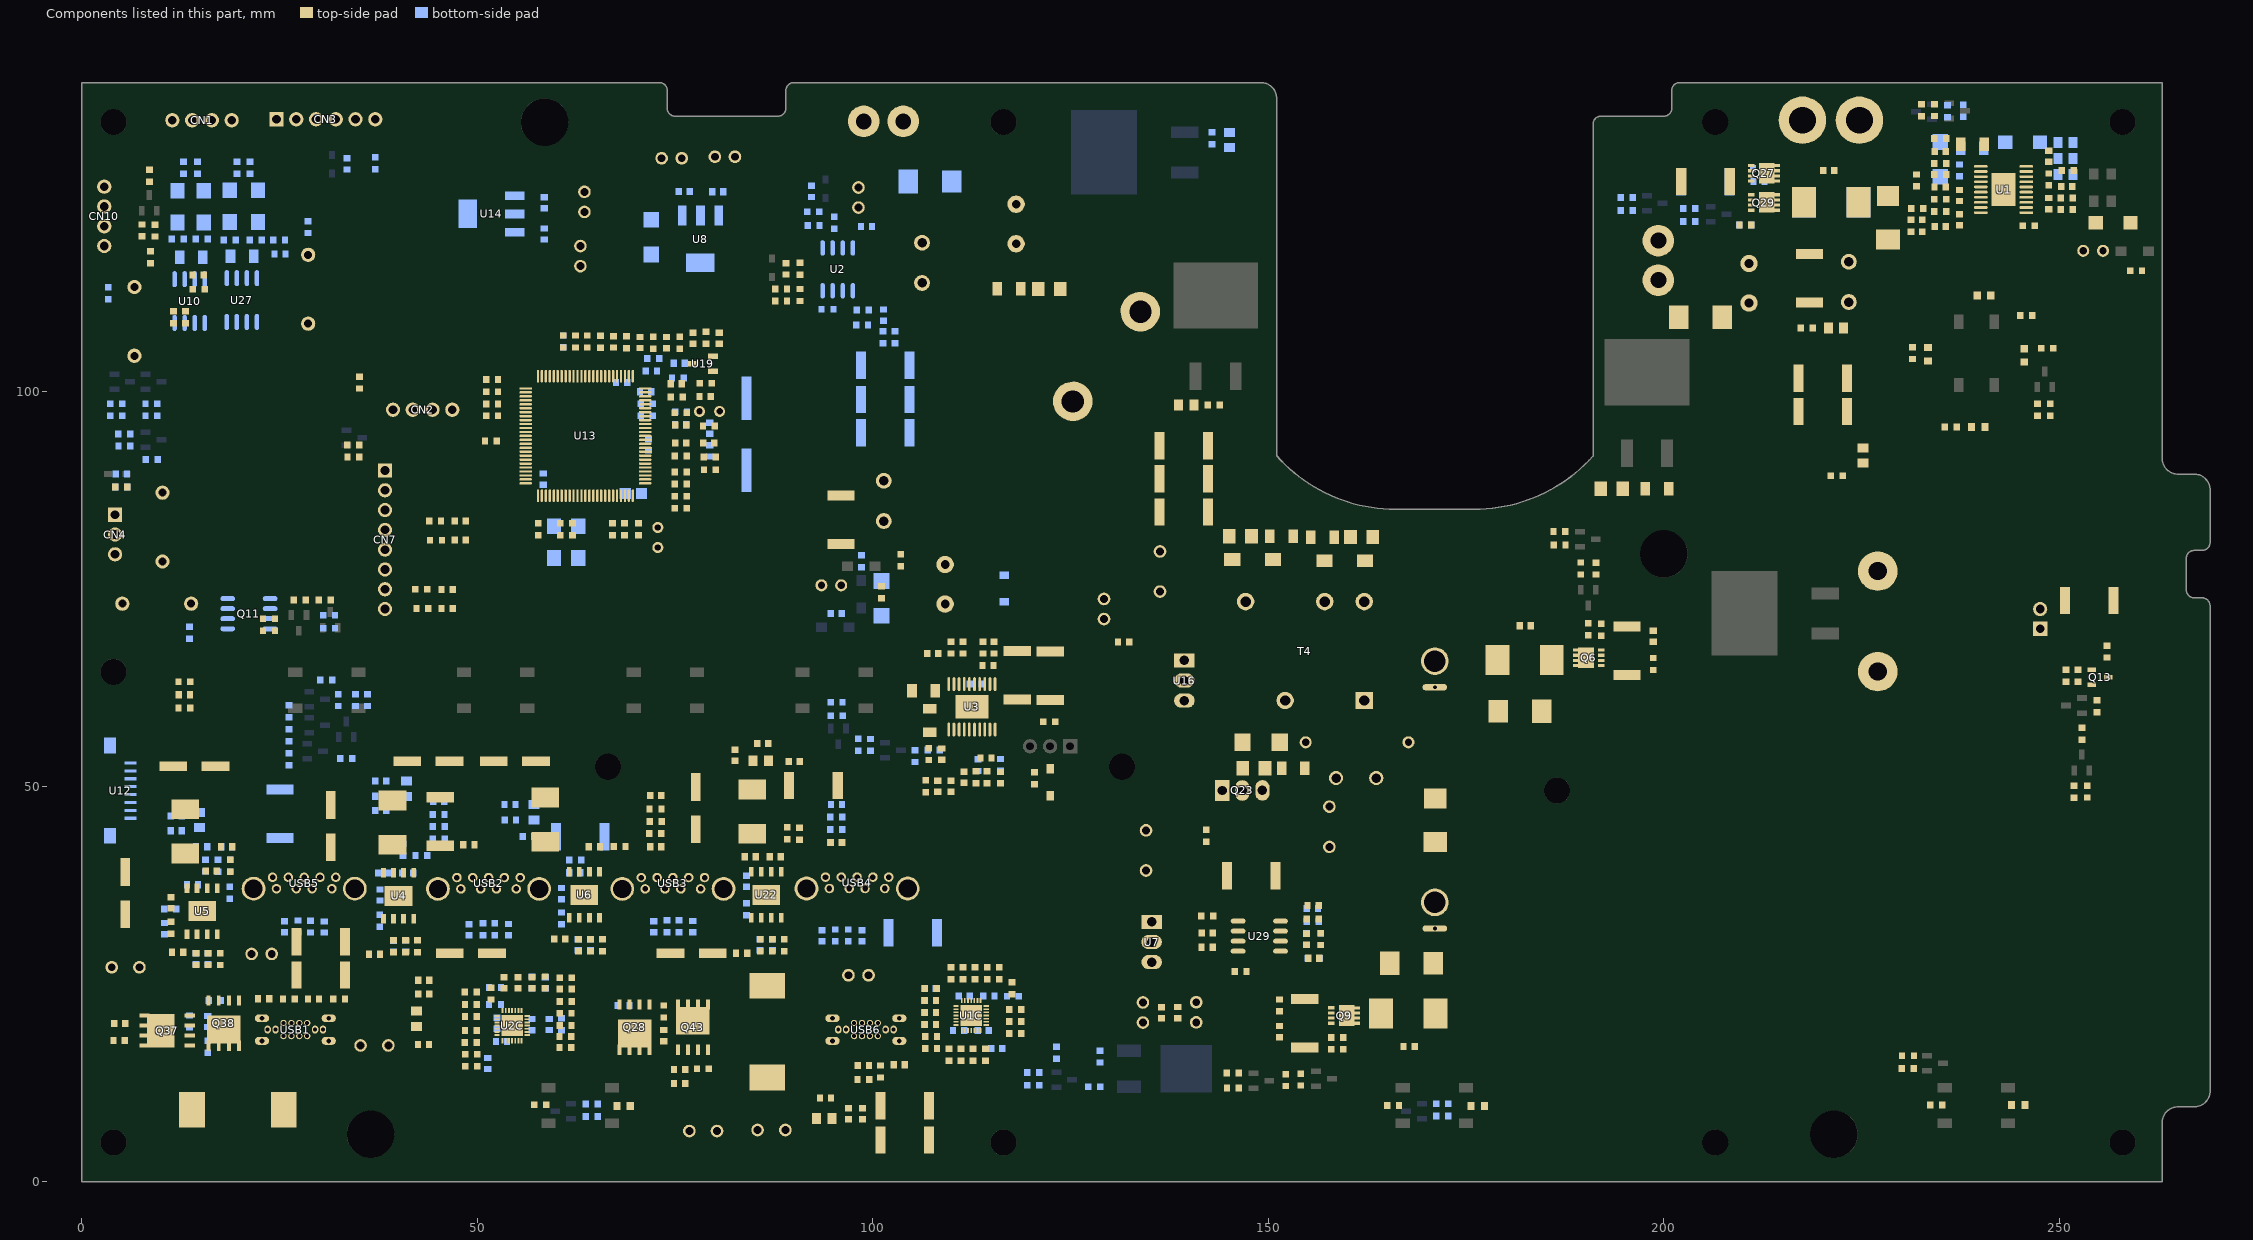
[diagram p0: the components of this part, seen from the top]
# Altium PCB MISC84402.PcbDoc (part 2 of 12)
Units mm, origin at the board's own origin, x right, y up, seen from the top; angles counter-clockwise.
Board outline 269.06 x 139 mm, 4 copper layers (TOP, GND02, PWR03, BOTTOM), stack 0.732 mm thick; 694 components, 428 nets, 1859 pads, 1384 vias.

## Components (designator, comment, footprint, x,y, rotation, side; value= is the part's Value field where it differs from the comment) (continued)
R13 "AC2512FK-073KL" R2512 118.238,64.049 r270 top
R14 "" R0603 113.03,51.181 r270 top
R15 "" R0603 109.855,67.564 r270 top
R16 "15K" RES-TH_BD3.3-L9.0-P13.00-D0.6 161.212,55.591 r0 top
R17 "1K" R0603 45.085,46.441 r0 bottom
R18 "0.01" R2512 220.109,97.409 r180 top
R19 "" RES-SMD_L6.4-W3.2-R2512 195.334,67.157 r0 top
R20 "49.9K" R0603 120.447,51.044 r90 top
R21 "" R0603 246.126,120.904 r180 top
R22 "" R0603 113.919,67.564 r270 top
R23 "2K" R0603 154.102,12.944 r90 top
R24 "1K" R0603 45.102,44.923 r180 bottom
R25 "" R0603 115.316,67.564 r270 top
R26 "" R2512 205.263,126.496 r0 top
R27 "" R0603 250.943,124.398 r180 top
R28 "" R2512 45.289,45.583 r90 top
R29 "" R0603 152.187,12.886 r270 top
R30 "1K" R0603 18.695,36.549 r90 bottom
R31 "" R2512 25.045,46.574 r90 bottom
R32 "2K" R0603 145.5,13.777 r0 top
R33 "" R0603 79.4,90.053 r0 top
R34 "" R0603 232.029,123.063 r0 top
R35 "2K" R0603 189.484,77.562 r90 top
R36 "" R0603 60.858,106.274 r270 bottom
R37 "" R0603 107.696,54.61 r0 bottom
R38 "" R0603 3.328,112.36 r90 bottom
R39 "" R0603 191.439,77.556 r90 top
R40 "2K" R0603 186.813,80.544 r0 top
R41 "" R2512 139.323,84.709 r0 top
R42 "" R0603 23.648,69.688 r180 top
R43 "" R0603 113.021,62.941 r180 bottom
R44 "" R0603 186.795,82.219 r180 top
R45 "" R2512 205.237,126.446 r0 bottom
R46 "" R0603 79.274,95.596 r0 top
R47 "1K" R0603 62.002,82.523 r90 top
R48 "" R0603 259.7,115.215 r180 top
R49 "" R0603 250.943,122.936 r180 top
R50 "AC2512FK-073KL" R2512 122.428,64.018 r90 top
R51 "2K" R0603 105.308,53.848 r90 bottom
R52 "" R0603 234.95,127.381 r0 top
R53 "" R0603 95.428,58.953 r0 bottom
R54 "" R1206 107.188,58.359 r90 top
R55 "" R0603 251.07,127.889 r180 top
R56 "" R0603 210.312,120.98 r0 top
R57 "100K" NTC 72.806,81.484 r90 top
R58 "1K" R0603 72.543,45.558 r0 top
R59 "" R2512 105.054,31.506 r180 bottom
R60 "" R0603 210.301,120.99 r0 bottom
R61 "" R0603 158.722,16.779 r180 top
R62 "1K" R0603 72.517,47.152 r180 top
R63 "" R0603 18.745,40.006 r270 bottom
R64 "2K" R0603 234.442,9.728 r0 top
R65 "10K" R0603 145.515,11.887 r180 top
R66 "" R0603 190.444,69.865 r270 top
R67 "1K" R0603 212.025,128.153 r0 bottom
R68 "" R0603 252.375,64.012 r90 top
R69 "1K" R0603 151.41,22.317 r270 top
R70 "1K" R0603 198.654,65.488 r90 top
R71 "" R0603 250.851,64.003 r90 top
R72 "" R0603 158.722,18.253 r0 top
R73 "2K" R0603 95.402,60.655 r180 bottom
R74 "" R0805 145.11,132.029 r270 bottom
R75 "" R0603 88.392,111.379 r180 top
R76 "" R0603 45.093,43.342 r180 bottom
R77 "1K" R0603 11.183,34.518 r0 bottom
R78 "2K" R0603 248.463,105.41 r0 top
R79 "2K" R0603 231.445,104.8 r270 top
R80 "" R0603 71.4,96.866 r180 bottom
R81 "100" R0603 40.92,29.818 r90 top
R82 "" R2512 63.018,43.653 r180 bottom
R83 "" R2512 92.482,50.13 r180 top
R84 "100" R0603 73.965,32.334 r90 bottom
R85 "1K" R0603 95.377,42.926 r180 bottom
R86 "" R0603 78.892,106.731 r90 top
R87 "" R0603 72.491,44.054 r0 top
R88 "36K" R0603 60.639,19.947 r90 bottom
R89 "100" R0603 39.396,29.818 r90 top
R90 "100" R0603 75.489,32.343 r90 bottom
R91 "" R0603 4.335,98.39 r180 bottom
R92 "100" R0603 28.905,32.292 r90 bottom
R93 "" R0603 8.789,98.39 r180 bottom
R94 "" R0603 51.85,98.339 r0 top
R95 "" R0603 36.094,60.925 r270 bottom
R96 "" R0603 95.352,44.552 r0 bottom
R97 "100" R0603 27.331,32.3 r90 bottom
R98 "2K" R0603 27.525,73.558 r0 top
R99 "1K" R0603 95.377,46.126 r0 bottom
R100 "10K" R0603 30.709,73.558 r180 top
R101 "" R0805 139.903,98.222 r180 top
R102 "100" R0603 52.197,31.957 r90 bottom
R103 "1K" R0603 18.745,39.999 r90 top
R104 "10K" R0603 98.146,55.27 r270 bottom
R105 "" R0603 5.368,93.056 r0 bottom
R106 "" R2512 101.582,98.933 r180 bottom
R107 "" R0603 90.805,115.443 r270 top
R108 "" R2512 101.582,94.742 r180 bottom
R109 "" R2512 101.582,103.251 r180 bottom
R110 "0.01" R2512 220.109,101.6 r180 top
R111 "100" R0603 62.764,29.945 r90 top
R112 "" R0603 98.628,108.356 r180 bottom
R113 "" R0603 32.503,23.114 r0 top
R114 "" R0603 26.171,23.114 r180 top
R115 "" R0603 98.806,12.954 r0 top
R116 "" R0603 100.965,13.97 r270 top
R117 "8.25K" R0603 146.481,26.594 r180 top
R118 "2K" R0603 236.271,95.453 r180 top
R119 "36K" R0603 117.704,23.485 r0 bottom
R120 "100" R0603 50.698,31.953 r90 bottom
R121 "" R0805 221.488,107.95 r0 top
R122 "" R0603 61.156,24.401 r0 top
R123 "100" R0603 96.891,31.174 r90 bottom
R124 "" R0603 256.047,67.065 r90 top
R125 "" R0805 225.171,91.567 r90 top
R126 "" R0603 68.479,22.317 r0 bottom
R127 "1K" R0603 117.602,24.511 r90 top
R128 "1K" R0603 117.991,21.809 r0 top
R129 "" R0603 117.991,20.285 r0 top
R130 "" R0603 117.991,18.761 r0 top
R131 "" R0603 78.512,14.316 r180 top
R132 "" R0603 17.479,28.18 r90 top
R133 "" R0603 42.444,29.818 r90 top
R134 "49.9K" R0603 156.617,30.707 r90 top
R135 "" R0603 65.812,29.945 r90 top
R136 "" R0603 231.267,120.904 r270 top
R137 "100" R0603 95.25,31.166 r90 bottom
R140 "" R0603 34.57,60.925 r270 bottom
R142 "" R0603 92.499,120.947 r0 bottom
R144 "" R0603 33.427,53.559 r0 bottom
R145 "" R0603 94.259,110.338 r0 bottom
R146 "" R0603 34.307,93.183 r180 top
R147 "1K" R0603 95.123,121.285 r90 bottom
R148 "" R0603 122.292,58.191 r0 top
R149 "" R0603 156.617,30.707 r90 bottom
R150 "" R0603 75.709,86.706 r0 top
R151 "" R0603 112.929,26.372 r90 top
R152 "" R0603 5.351,94.58 r180 bottom
R153 "" R0603 26.188,53.432 r270 bottom
R154 "" R0603 11.583,109.32 r90 top
R155 "20K" R0603 155.728,28.286 r0 bottom
R156 "" R0603 13.107,109.32 r90 top
R157 "" R0603 35.078,101.065 r270 top
R158 "" R0603 28.601,120.733 r270 bottom
R159 "1K" R0603 4.352,96.866 r180 bottom
R160 "" R0603 107.329,24.476 r0 top
R161 "NC" R0603 114.453,26.372 r90 top
R162 "NC" R0603 115.977,26.372 r90 top
R163 "100K" NTC 79.35,97.424 r0 top
R164 "" R0603 107.225,22.952 r0 bottom
R165 "1K" R0603 8.814,91.33 r180 bottom
R166 "" R0603 107.225,21.428 r0 bottom
R167 "" R0603 107.225,19.904 r0 bottom
R168 "" R0603 154.839,30.707 r270 bottom
R169 "0.01" R2512 104.021,5.299 r0 top
R170 "" R0603 107.349,18.38 r0 top
R172 "" R0603 192.095,69.815 r270 top
R173 "" R0603 107.349,16.856 r0 top
R174 "" R0603 73.559,21.555 r90 top
R175 "" R0603 109.627,16.085 r90 top
R176 "1K" R0603 34.325,91.659 r180 top
R177 "10K" R0603 195.307,124.45 r180 bottom
R178 "" R0603 111.151,16.102 r90 top
R179 "" R0603 112.675,16.094 r90 top
R180 "" R0603 26.188,59.528 r270 bottom
R181 "NC" R0603 114.223,16.097 r270 top
R182 "NC" R0603 61.148,19.804 r0 top
R183 "" R0603 23.648,71.212 r180 top
R184 "1K" R0603 8.789,96.866 r180 bottom
R185 "NC" R0603 61.148,21.328 r0 top
R186 "2K" R0603 31.242,70.002 r180 bottom
R187 "2K" R0603 245.821,109.55 r0 top
R188 "" R0603 26.188,56.48 r270 bottom
R189 "" R0603 61.155,22.825 r0 top
R190 "" R0603 155.625,32.944 r180 bottom
R191 "2K" R0603 195.295,122.834 r0 bottom
R192 "" R0603 15.147,119.218 r0 bottom
R193 "10K" R0603 31.242,71.644 r0 bottom
R194 "2K" R0603 57.937,9.754 r0 top
R195 "2K" R0603 165.76,9.652 r0 top
R196 "" R0603 111.405,26.372 r270 top
R197 "" R0603 13.615,69.434 r90 bottom
R198 "" R1206 117.221,112.903 r180 top
R199 "1K" R0603 61.13,18.381 r0 top
R200 "1K" R0603 61.13,16.984 r0 top
R201 "" R0603 49.218,14.622 r180 top
R202 "" R0603 49.209,16.146 r180 top
R203 "" R0603 58.573,25.229 r270 top
R204 "" R0603 52.223,24.603 r0 bottom
R205 "" R0603 56.922,25.229 r270 bottom
R206 "" R1206 199.119,87.63 r0 top
R207 "" R0603 44.641,83.569 r180 top
R208 "" R0603 52.223,22.444 r0 bottom
R209 "" R0603 16.79,22.952 r0 bottom
R210 "" R0603 116.154,52.722 r270 bottom
R211 "" R0603 51.715,23.824 r270 top
R212 "" R0603 13.615,20.293 r270 bottom
R213 "" R0603 49.168,24.003 r0 top
R214 "" R0603 49.183,22.444 r0 top
R215 "" R0603 49.183,20.92 r0 top
R216 "" R0603 49.183,19.142 r0 top
R217 "" R0603 51.715,93.691 r180 top
R218 "NC" R0603 49.165,17.638 r180 top
R219 "" R0603 75.709,88.23 r0 top
R220 "120" R1206 13.824,116.932 r0 bottom
R221 "" R0603 75.709,89.754 r0 top
R222 "" R0603 57.684,82.506 r270 top
R223 "" R0603 107.061,54.102 r90 top
R224 "" R0603 62.383,106.264 r270 top
R225 "" R0603 14.631,128.226 r90 bottom
R226 "" R0603 15.901,17.11 r270 bottom
R227 "" RES-SMD_L6.4-W3.2-R2512 154.618,20.066 r180 top
R228 "" R0603 70.384,82.523 r270 top
R229 "" R0603 14.766,112.868 r180 top
R230 "" R0603 21.988,119.091 r0 bottom
R231 "" R0603 24.918,119.091 r0 bottom
R232 "" R0603 12.099,119.218 r0 bottom
R233 "" R0603 21.235,128.226 r90 bottom
R234 "" R0603 12.853,128.243 r90 bottom
R235 "" R0603 19.584,128.226 r90 bottom
R237 "" R0603 71.4,98.39 r0 bottom
R238 "100" R0603 64.288,29.945 r90 top
R239 "120" R1206 20.264,117.059 r180 bottom
R240 "22" R0603 142.266,33.62 r180 top
R241 "" R0603 90.703,44.028 r270 top
R242 "100" R0603 15.955,28.18 r90 top
R243 "100" R0603 14.431,28.18 r90 top
R244 "" R0603 18.686,119.091 r0 bottom
R245 "100" R0603 87.275,29.945 r90 top
R246 "" R0603 51.85,99.914 r0 top
R247 "100" R0603 85.751,29.945 r90 top
R248 "36K" R0603 232.664,120.904 r270 top
R249 "" R0603 51.85,101.438 r0 top
R250 "" R0603 67.082,82.523 r270 top
R251 "" R0603 68.606,82.523 r270 top
R252 "" R0603 75.709,85.182 r0 top
R253 "" R0603 218.059,107.95 r0 top
R254 "" R0603 44.764,81.128 r180 top
R255 "" R0603 42.917,74.93 r180 top
R256 "" R0603 79.384,91.659 r180 top
R257 "" R0603 75.718,97.247 r180 top
R258 "1K" R0603 155.601,33.239 r180 top
R259 "" R0603 221.86,89.281 r0 top
R260 "" R0603 142.875,131.953 r90 bottom
R261 "" R0603 143.078,98.222 r180 top
R262 "0.01" R2512 30.208,30.353 r180 top
R264 "" R0603 43.044,72.517 r180 top
R265 "" R0603 142.139,43.78 r90 top
R266 "0.01" R2512 104.021,9.617 r0 top
R267 "0.01" R2512 30.208,26.162 r180 top
R268 "" R0603 101.295,106.807 r90 bottom
R269 "" R0603 63.881,106.264 r270 top
R270 "" R0603 37.084,128.787 r270 bottom
R271 "1K" R0603 92.465,122.666 r180 bottom
R272 "10K" R0603 253.534,49.361 r270 top
R273 "" R0603 11.261,32.148 r90 top
R274 "NC" R0603 248.666,126.746 r270 top
R276 "" R0603 4.979,87.849 r0 bottom
R277 "" R0603 37.659,33.037 r90 bottom
R278 "" R0603 60.621,33.316 r90 bottom
R279 "" R0603 84.039,34.485 r90 bottom
R280 "" R0603 75.192,99.247 r180 top
R281 "" R0603 102.794,106.782 r90 bottom
R282 "" R0603 78.859,100.981 r0 top
R283 "" R0603 51.85,96.866 r0 top
R284 "" R0603 75.353,101.66 r0 bottom
R285 "" R0603 72.221,104.131 r180 bottom
R286 "" R0603 75.751,97.374 r180 bottom
R287 "2K" R0603 251.876,49.344 r90 top
R288 "10K" R0603 252.866,56.684 r90 top
R289 "2K" R0603 254.778,60.13 r270 top
R290 "" R0603 98.704,110.236 r180 bottom
R291 "2K" R0603 99.704,55.253 r270 bottom
R292 "" R0603 88.799,29.937 r90 top
R293 "" R0603 75.718,91.786 r0 top
R294 "" R0603 90.805,112.141 r270 top
R295 "1K" R0603 88.392,112.903 r0 top
R296 "2K" R0603 231.927,126.619 r90 top
R297 "10K" R0603 234.204,135.517 r270 top
R298 "" R0603 4.97,87.849 r0 top
R302 "2K" R0603 232.572,135.501 r90 top
R306 "" R0603 234.95,122.682 r180 top
R307 "" R0603 61.156,25.823 r180 top
R308 "10K" R0603 237.862,135.424 r90 bottom
R309 "" R0603 109.881,26.389 r270 top
R314 "2K" R0603 235.881,135.374 r90 bottom
R316 "0.15" R2512 147.836,38.7 r0 top
R317 "" R0603 75.574,106.113 r90 top
R319 "" R0603 32.411,60.925 r90 bottom
R320 "" R0603 30.887,63.465 r0 bottom
R321 "" R0603 12.954,63.246 r180 top
R322 "" R0603 12.954,59.944 r0 top
R323 "10K" R0603 230.869,15.96 r180 top
R324 "1K" R0603 60.478,82.515 r90 top
R325 "2K" R0603 230.852,14.342 r0 top
R326 "" R0603 98.552,78.486 r90 bottom
R327 "" R0805 251.079,127.381 r180 bottom
R328 "" R0805 251.079,131.445 r180 bottom
R329 "" R0805 251.079,129.413 r180 bottom
R330 "" R1206 238.989,130.708 r0 bottom
R331 "" R1206 106.426,62.103 r0 top
R332 "10K" R0603 248.86,97.621 r270 top
R333 "2K" R0603 247.227,97.629 r90 top
R334 "10K" R0603 64.457,9.864 r0 bottom
R335 "2K" R0603 64.448,8.297 r180 bottom
R336 "10K" R0603 172,8.34 r0 bottom
R337 "2K" R0603 171.992,9.897 r180 bottom
R338 "" R0603 123.199,16.341 r270 bottom
R339 "" R0603 89.179,44.104 r270 top
R340 "" R0603 62.357,40.726 r0 bottom
R341 "" R0603 67.97,42.428 r180 top
R342 "" R0603 40.599,41.987 r270 bottom
R343 "" R0603 42.926,41.26 r180 bottom
R344 "" R0603 17.221,39.973 r270 bottom
R345 "" R0603 15.621,40.006 r270 bottom
R348 "" R0603 127.982,12.049 r0 bottom
R349 "" R0603 120.277,13.859 r180 bottom
R350 "20K" R0603 120.261,12.227 r0 bottom
R351 "20K" R0603 128.711,15.858 r270 bottom
R352 "10K" R0603 203.217,121.421 r0 bottom
R353 "2K" R0603 203.217,123.072 r0 bottom
R354 "" R0603 72.221,106.087 r90 top
R355 "" R0603 68.843,106.164 r90 top
R356 "" R0603 65.541,106.24 r90 top
R357 "" R0603 234.933,124.241 r180 top
R358 "" R2512 95.97,83.735 r90 top
R359 "" R1206 151.672,81.645 r180 top
R360 "" R1206 156.837,81.525 r0 top
R361 "" R1206 153.145,52.308 r180 top
R362 "" R0603 103.521,78.621 r270 top
R363 "2K" R0603 8.551,127.212 r270 top
R364 "2K" R0603 9.229,120.286 r90 top
R365 "10K" R0603 7.585,120.303 r270 top
R366 "" R0603 8.652,116.925 r270 top
R367 "AC2512FK-073KL" R2512 218.405,114.258 r270 top
R368 "15" r2512 253.805,73.517 r180 top
T4 "EE22 4:5" "EE22 4:5NEW" 154.625,67.121 r180 bottom
U1 "LM5116MHX" HTSSOP-20_L6.5-W4.4-P0.65-LS6.4-BL-EP 242.951,125.476 r270 top
U1C "Value" QFN-28_L4.0-W4.0-P0.40-BL-EP 112.421,21.047 r270 top
U2 "EG358" SOIC-8_L5.0-W4.0-P1.27-LS6.0-BL 94.869,114.3 r180 bottom
U2C "Value" QFN-28_L4.0-W4.0-P0.40-BL-EP 54.382,19.777 r180 top
U3 "LM5116MHX" HTSSOP-20_L6.5-W4.4-P0.65-LS6.4-BL-EP 112.522,60.071 r0 top
U4 "SW3521" ESOP-8_L4.9-W3.9-P1.27-LS6.0-BL-EP 40.031,36.16 r180 top
U5 "SW3521" ESOP-8_L4.9-W3.9-P1.27-LS6.0-BL-EP 15.193,34.255 r180 top
U6 "SW3521" ESOP-8_L4.9-W3.9-P1.27-LS6.0-BL-EP 63.526,36.287 r180 top
U7 "L7805CV-DG" TO-220-3_L10.0-W4.5-P2.54-L 135.239,30.336 r270 bottom
U8 "LM1117S-3.3" SOT-223-3_L6.5-W3.4-P2.30-LS7.0-BR 78.198,119.211 r90 bottom
U10 "WS3085" SOP-8_L5.0-W4.0-P1.27-LS6.0-BL 13.615,111.37 r180 bottom
U12 "KH-FG1.0-H2.0-8PIN" FPC-SMD_KH-FG1.0-H2.0-8PIN 4.826,49.479 r90 bottom
U13 "GD32F103VCT6" LQFP-100_L14.0-W14.0-P0.50-LS16.0-BL 63.653,94.326 r90 top
U14 "LM1117S-3.3" SOT-223-3_L6.5-W3.4-P2.30-LS7.0-BR 51.751,122.393 r0 bottom
U16 "L7812CV_C347292" TO-220-3_L10.0-W4.5-P2.54-L 139.383,63.398 r270 bottom
U19 "TL431_C2688223" SOT-23-3_L2.9-W1.6-P1.90-LS2.8-BR-CW 78.512,103.47 r0 top
U22 "SW3521" ESOP-8_L4.9-W3.9-P1.27-LS6.0-BL-EP 86.513,36.287 r180 top
U27 "WS3085" SOP-8_L5.0-W4.0-P1.27-LS6.0-BL 20.219,111.497 r180 bottom
U29 "UC2845BD1013TR" SOP-8_L4.9-W3.9-P1.27-LS6.0-BL 148.854,31.08 r90 top
USB1 "TYPE-C2022512" NEW_TYPEC 26.98,19.269 r180 top
USB2 "916-252A205IY30200" USB-A-TH_916-252A205IY30200 51.41,37.772 r0 top locked
USB3 "916-252A205IY30200" USB-A-TH_916-252A205IY30200 74.715,37.772 r0 top
USB4 "916-252A205IY30200" USB-A-TH_916-252A205IY30200 98.007,37.823 r0 top
USB5 "916-252A205IY30200" USB-A-TH_916-252A205IY30200 28.098,37.797 r0 top locked
USB6 "TYPE-C2022512" NEW_TYPEC 99.121,19.269 r180 top
X1 "8MHz" HC-49S_L11.4-W4.8 84.023,94.52 r90 bottom

## Footprints (in the part's own frame and the unit in brackets; to place one, negate y for a bottom-side part, rotate by r counter-clockwise, add the part's x,y. Pads: shape width x height; smd on the part's side, far side on the other; paste and mask are expansions set on the pad)
C0603 [mm]
  rect 0.8x0.9 smd: 1(-0.7,0) 2(0.7,0)
  silkscreen extent -1.41,-0.71 1.39,0.72
C0805 [mm]
  rect 1.41x1.35 smd: 1(-1.03,0) 2(1.03,0)
  silkscreen extent -1.96,-0.9 1.96,0.9
C1206 [mm] "Chip Capacitor; Body 3.2 x 1.6 mm (LxW typ)"
  rect 1.6x1.8 smd: 1(-1.4,0) 2(1.4,0)
  silkscreen extent -0.3,-0.8 0.3,0.8
CAP-SMD_BD6.3-L6.6-W6.6-FD [mm]
  rect 3.5x1.2 smd: 1(-2.67,0) 2(2.67,0)
  silkscreen extent -3.38,-3.38 3.38,3.38
CAP-TH_BD5.0-P2.5-D0.5-FD [mil]
  round 60 hole 36: 1(-49.21,0) 2(49.21,0)
  silkscreen extent -98,-98 98,98
CAP-TH_BD6.3-P2.50-D1.0-FD [mm]
  round 1.6 hole 1: 1(-1.27,0) 2(1.27,0)
  silkscreen extent -3.15,-3.15 3.15,3.15
CAP-TH_BD8.0-P3.50-D0.6-FD [mm]
  round 1.6 hole 1: 1(-1.75,0) 2(1.75,0)
  silkscreen extent -3.96,-4 4.04,4
CAP-TH_BD10.0-P5.00-D1.0-FD [mm]
  round 1.6 hole 1: 1(-2.54,0) 2(2.54,0)
  silkscreen extent -5,-5 5.08,5
CAP-TH_BD12.5-P5.00-D0.6-FD [mm]
  round 2.2 hole 1.1: 1(-2.5,0) 2(2.5,0)
  silkscreen extent -6.25,-6.25 6.25,6.25
CAP-TH_BD13.0-P5.00-D1.2-FD [mm]
  round 2 hole 1.2: 1(-2.539,0) 2(2.541,0)
  silkscreen extent -6.5,-6.5 6.5,6.5
CAP-TH_L8.0-W4.0-P5.00-D1.2 [mm]
  round 1.8 hole 1.2: 1(-2.54,0) 2(2.54,0)
  silkscreen extent -4,-2 4,2
CONN-TH_2P-P2.50_HX25003-2A [mm]
  rect 1.8x1.8 hole 1.1: 1(-1.25,0.646)
  round 1.8 hole 1.1: 2(1.25,0.646)
  silkscreen extent -3.75,-3.05 3.75,3.05
CONN-TH_3P-P2.50_B3B-XH-A-LF-SN [mm]
  rect 1.8x1.8 hole 1.1: 1(-2.5,0)
  round 1.8 hole 1.1: 2(0,0) 3(2.5,0)
  silkscreen extent -5,-3.5 5,2.5
CONN-TH_4P-P2.50_HX25003-4A [mm]
  round 1.8 hole 1.1: 1(-3.75,0.645) 2(-1.25,0.645) 3(1.25,0.645) 4(3.75,0.645)
  silkscreen extent -6.25,-3.06 6.25,3.06
CONN-TH_6P-P2.50_B6B-XH-A-LF-SN [mm]
  rect 1.8x1.8 hole 1.1: 1(-6.251,0.501)
  round 1.8 hole 1.1: 2(-3.749,0.499) 3(-1.249,0.499) 4(1.251,0.499) 5(3.751,0.499) 6(6.251,0.499)
  silkscreen extent -8.75,-3 8.75,3
CONN-TH_8P-P2.50_HX25003-8A [mm]
  rect 1.8x1.8 hole 1.1: 1(8.75,0.646)
  round 1.8 hole 1.1: 2(6.25,0.646) 3(3.75,0.646) 4(1.25,0.646) 5(-1.25,0.646) 6(-3.75,0.646) 7(-6.25,0.646) 8(-8.75,0.646)
  silkscreen extent -11.25,-3.05 11.25,3.05
CONN-TH_XT30UPB-F-W [mm]
  round 4 hole 2: 1(-2.5,0) 2(2.5,0)
CONN-TH_XT60UPB-F-W [mm]
  round 6 hole 3.4: 1(3.6,0) 2(-3.6,0)
DC5521 [mm]
  round 3.5 hole 2.7: 1(0,0)
  oval 3.1x0.8 hole 0.5 slot 2.7 at 0 deg: 2(0,-3.302)
  silkscreen extent -4,-4 4,4
DO-41_BD2.4-L4.7-P8.70-D0.9-RD [mm]
  round 1.8 hole 1: 1(-4.35,0) 2(4.35,0)
  silkscreen extent -2.6,-1.4 2.6,1.4
"EE22 4:5NEW" [mm]
  rect 2.2x2.2 hole 1.3: 1(-7.5,-6.25)
  round 2.2 hole 1.3: 3(2.5,-6.25) 5(7.5,6.25) 7(-2.5,6.25) 8(-7.5,6.25)
  silkscreen extent -11,-8.5 11,8.5
ESOP-8_L4.9-W3.9-P1.27-LS6.0-BL-EP [mm]
  rect 0.6x1.2 smd: 1(-1.905,-2.908) 2(-0.635,-2.908) 3(0.635,-2.908) 4(1.905,-2.908) 5(1.905,2.908) 6(0.635,2.908) 7(-0.635,2.908) 8(-1.905,2.908)
  rect 3.5x2.5 smd: 9(0,0)
  silkscreen extent -3.2,-2.67 2.55,2.05
FPC-SMD_KH-FG1.0-H2.0-8PIN [mm]
  rect 0.4x1.5 smd: 1(3.5,1.3) 2(2.5,1.3) 3(1.5,1.3) 4(0.5,1.3) 5(-0.5,1.3) 6(-1.5,1.3) 7(-2.5,1.3) 8(-3.5,1.3)
  rect 2x1.5 smd: 9(-5.7,-1.3) 10(5.7,-1.3)
  silkscreen extent -6.45,-4.4 6.5,1.49
FUSE-SMD_L6.1-W2.5#1 [mm]
  rect 2.5x3 smd: 1(-2.75,0)
  rect 2.5x2.83 smd: 2(2.75,0)
  silkscreen extent -1.02,-0.51 1.02,0.51
FUSE-SMD_L6.1-W2.5#2 [mm]
  rect 2.5x3 smd: 1(-2.75,0) 2(2.75,0)
  silkscreen extent -1.02,-0.51 1.02,0.51
HC-49S_L11.4-W4.8 [mm]
  rect 5.5x1.3 smd: 1(4.553,0) 2(-4.553,0)
  silkscreen extent -5.71,-2.41 5.71,2.41
HTSSOP-20_L6.5-W4.4-P0.65-LS6.4-BL-EP [mm]
  oval 0.343x1.747 smd: 1(-2.925,-2.873) 2(-2.275,-2.873) 3(-1.625,-2.873) 4(-0.975,-2.873) 5(-0.325,-2.873) 6(0.325,-2.873) 7(0.975,-2.873) 8(1.625,-2.873) 9(2.275,-2.873) 10(2.925,-2.873) 11(2.925,2.873) 12(2.275,2.873) 13(1.625,2.873) 14(0.975,2.873) 15(0.325,2.873) 16(-0.325,2.873) 17(-0.975,2.873) 18(-1.625,2.873) 19(-2.275,2.873) 20(-2.925,2.873)
  rect 4.2x3 smd: 21(0,0)
  silkscreen extent -3.7,-3.02 3.33,1.77
IND-SMD_L7.1-W6.8 [mm]
  rect 2.5x3.5 smd: 1(-2.8,0) 2(2.8,0)
  silkscreen extent -3.7,-3.4 3.7,3.4
IND-SMD_L13.8-W12.6_YSPI13XX [mm]
  rect 3.25x4.5 smd: 1(-5.8,0) 2(5.8,0)
  silkscreen extent -6.3,-6.3 6.3,6.3
IND-TH_CS270026-W280M-N [mm]
  round 5 hole 2.8: 1(-7.096,0) 2(7.096,0)
  silkscreen extent -8.61,-18 27.38,18
IND-TH_CS270026-W560M-N [mm]
  round 5 hole 2.3 slot 2.305 at 0 deg: 1(6.35,0) 2(-6.35,0)
  silkscreen extent -27.78,-17.51 7.43,17.51
L0805 [mm]
  rect 1.133x1.377 smd: 1(-0.966,0) 2(0.966,0)
  silkscreen extent -1.95,-1.02 1.86,1.02
LED0603_RED [mm]
  rect 0.9x1 smd: 1(-0.85,0) 2(0.85,0)
  silkscreen extent -1.54,-0.73 1.75,0.73
LQFP-100_L14.0-W14.0-P0.50-LS16.0-BL [mm]
  oval 0.3x1.6 smd: 1(-6,-7.55) 2(-5.5,-7.55) 3(-5,-7.55) 4(-4.5,-7.55) 5(-4,-7.55) 6(-3.5,-7.55) 7(-3,-7.55) 8(-2.5,-7.55) 9(-2,-7.55) 10(-1.5,-7.55) 11(-1,-7.55) 12(-0.5,-7.55) 13(0,-7.55) 14(0.5,-7.55) 15(1,-7.55) 16(1.5,-7.55) 17(2,-7.55) 18(2.5,-7.55) 19(3,-7.55) 20(3.5,-7.55) 21(4,-7.55) 22(4.5,-7.55) 23(5,-7.55) 24(5.5,-7.55) 25(6,-7.55) 51(6,7.55) 52(5.5,7.55) 53(5,7.55) 54(4.5,7.55) 55(4,7.55) 56(3.5,7.55) 57(3,7.55) 58(2.5,7.55) 59(2,7.55) 60(1.5,7.55) 61(1,7.55) 62(0.5,7.55) 63(0,7.55) 64(-0.5,7.55) 65(-1,7.55) 66(-1.5,7.55) 67(-2,7.55) 68(-2.5,7.55) 69(-3,7.55) 70(-3.5,7.55) 71(-4,7.55) 72(-4.5,7.55) 73(-5,7.55) 74(-5.5,7.55) 75(-6,7.55)
  oval 1.6x0.3 smd: 26(7.55,-6) 27(7.55,-5.5) 28(7.55,-5) 29(7.55,-4.5) 30(7.55,-4) 31(7.55,-3.5) 32(7.55,-3) 33(7.55,-2.5) 34(7.55,-2) 35(7.55,-1.5) 36(7.55,-1) 37(7.55,-0.5) 38(7.55,0) 39(7.55,0.5) 40(7.55,1) 41(7.55,1.5) 42(7.55,2) 43(7.55,2.5) 44(7.55,3) 45(7.55,3.5) 46(7.55,4) 47(7.55,4.5) 48(7.55,5) 49(7.55,5.5) 50(7.55,6) 76(-7.55,6) 77(-7.55,5.5) 78(-7.55,5) 79(-7.55,4.5) 80(-7.55,4) 81(-7.55,3.5) 82(-7.55,3) 83(-7.55,2.5) 84(-7.55,2) 85(-7.55,1.5) 86(-7.55,1) 87(-7.55,0.5) 88(-7.55,0) 89(-7.55,-0.5) 90(-7.55,-1) 91(-7.55,-1.5) 92(-7.55,-2) 93(-7.55,-2.5) 94(-7.55,-3) 95(-7.55,-3.5) 96(-7.55,-4) 97(-7.55,-4.5) 98(-7.55,-5) 99(-7.55,-5.5) 100(-7.55,-6)
  silkscreen extent -7.03,-8 6.25,6.25
NEW_TYPEC [mm]
  oval 1.8x1 hole 0.6 slot 1.3 at 0 deg: 17(-4.225,-1.43) 17(-4.225,1.43) 17(4.225,-1.43) 17(4.225,1.43)
  oval 0.8x1 hole 0.5 slot 0.7 at 90 deg: A1(-3.5,0) A4(-2.5,0) A9(2.5,0) A12(3.5,0)
  round 0.8 hole 0.5: A5(-1.5,0.825) A6(-0.5,0.825) A7(0.5,0.825) A8(1.5,0.825) B5(1.5,-0.825) B6(0.5,-0.825) B7(-0.5,-0.825) B8(-1.5,-0.825)
  silkscreen extent -4.21,-1.46 4.29,1.46
NTC [mm]
  round 1.4 hole 0.8: 1(-1.27,0) 2(1.27,0)
PDFN-8_L3.1-W3.1-P0.65-LS3.4-BL [mm]
  rect 0.4x0.8 smd: 1(-0.975,-1.6) 2(-0.325,-1.6) 3(0.325,-1.6) 4(0.975,-1.6) 5(0.975,1.6) 6(0.325,1.6) 7(-0.325,1.6) 8(-0.975,1.6)
  rect 2.6x2 smd: 9(-0.005,0.35)
  silkscreen extent -1.59,-2.41 1.56,1.55
POWERPAK-SO-8_L6.2-W5.2-P1.27-BR-EP [mm]
  rect 1.3x0.5 smd: 1(2.858,-1.905) 2(2.858,-0.635) 3(2.858,0.635) 4(2.858,1.905) 5(-2.858,1.905) 6(-2.858,0.635) 7(-2.858,-0.635) 8(-2.858,-1.905)
  rect 3.5x4.25 smd: 8(-0.813,0)
  silkscreen extent -3,-2.54 4,2.54
QFN-28_L4.0-W4.0-P0.40-BL-EP [mm]
  rect 0.224x0.665 smd: 1(-1.2,-1.907) 2(-0.8,-1.907) 3(-0.4,-1.907) 4(0,-1.907) 5(0.4,-1.907) 6(0.8,-1.907) 7(1.2,-1.907) 15(1.2,1.908) 16(0.8,1.908) 17(0.4,1.908) 18(0,1.908) 19(-0.4,1.908) 20(-0.8,1.908) 21(-1.2,1.908)
  rect 0.665x0.224 smd: 8(1.907,-1.2) 9(1.907,-0.8) 10(1.907,-0.4) 11(1.907,0) 12(1.907,0.4) 13(1.907,0.8) 14(1.907,1.2) 22(-1.907,1.2) 23(-1.907,0.8) 24(-1.907,0.4) 25(-1.907,0) 26(-1.907,-0.4) 27(-1.907,-0.8) 28(-1.907,-1.2)
  rect 2.7x2.7 smd: 29(0,0)
  silkscreen extent -2.08,-2.61 2.08,2.08
R0603 [mm]
  rect 0.806x0.864 smd: 1(-0.753,0) 2(0.753,0)
  silkscreen extent -1.39,-0.66 1.39,0.66
R0805 [mm]
  rect 1.133x1.377 smd: 1(-0.678,0) 2(1.254,0)
  silkscreen extent -1.47,-0.92 2.05,0.92
R1206 [mm]
  rect 1.208x1.701 smd: 1(-1.479,0) 2(1.479,0)
  silkscreen extent -2.31,-1.08 2.31,1.08
R2512 [mm]
  rect 1.283x3.456 smd: 1(-3.066,0) 2(3.066,0)
  silkscreen extent -3.94,-1.96 3.94,1.96
r2512 [mm]
  rect 1.283x3.456 smd: 1(-3.066,0) 2(3.066,0)
  silkscreen extent -3.94,-1.96 3.94,1.96
RES-SMD_L6.4-W3.2-R2512 [mm]
  rect 3.456x1.283 smd: 1(0,3.066) 2(0,-3.066)
  silkscreen extent -1.96,-3.94 1.96,3.94
RES-TH_BD3.3-L9.0-P13.00-D0.6 [mil]
  round 60 hole 36: 1(-255.91,0) 2(255.9,0)
  silkscreen extent -210,-65 210,65
SC-59-3_L2.9-W1.5-P0.95-LS2.5-BR [mm]
  rect 1.058x0.532 smd: 1(1.041,-0.95) 2(1.041,0.95) 3(-1.041,0)
  silkscreen extent -0.79,-1.53 0.79,1.53
SMA_L4.3-W2.5-LS5.0-BI [mm]
  rect 2x1.8 smd: 1(-2,0) 2(2,0)
  silkscreen extent -2.3,-1.4 2.3,1.4
SMA_L4.3-W2.6-LS5.2-RD [mm]
  rect 2x2 smd: 1(-2.2,0) 2(2.2,0)
  silkscreen extent -2.98,-1.5 2.6,1.5
SMA_L4.4-W2.6-LS5.0-RD [mm]
  rect 1.8x1.7 smd: 1(-2.192,0) 2(2.192,0)
  silkscreen extent -3.11,-1.48 2.73,1.48
SMA_L4.4-W2.8-LS5.4-RD [mm]
  rect 2.046x1.62 smd: 1(-2.566,0) 2(2.565,0)
  silkscreen extent -3.08,-1.44 2.7,1.44
SMB_L4.6-W3.6-LS5.3-RD [mm]
  rect 2.047x2.192 smd: 1(-2.361,0) 2(2.361,0)
  silkscreen extent -3.12,-1.96 2.74,1.96
SMC_L7.1-W6.2-LS8.1-R-RD [mm]
  rect 3.03x3.82 smd: 1(3.435,0) 2(-3.435,0)
  silkscreen extent -3.6,-3.11 3.6,3.11
SOD-123_L2.7-W1.6-LS3.7-RD-1 [mm]
  rect 1.2x0.95 smd: 1(-1.7,0) 2(1.7,0)
  silkscreen extent -1.81,-0.98 1.35,0.98
SOD-123_L2.8-W1.8-LS3.7-RD [mm]
  rect 0.95x1.15 smd: 1(-1.693,0) 2(1.693,0)
  silkscreen extent -1.63,-0.94 1.41,0.94